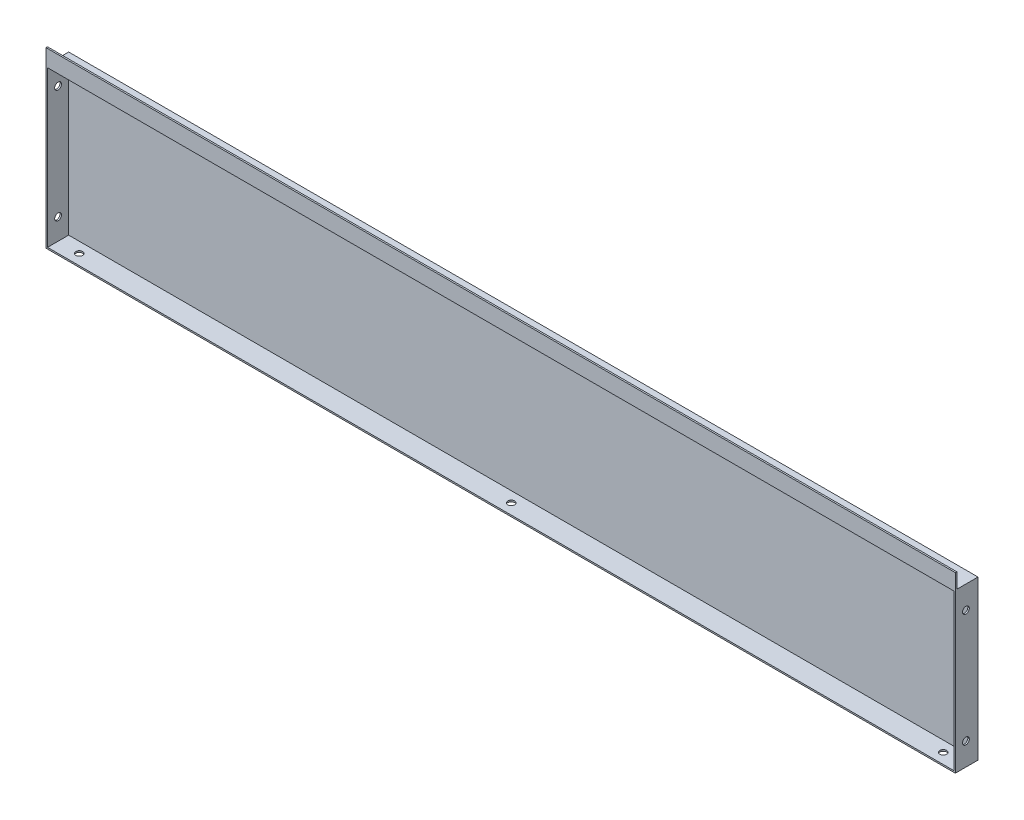
from build123d import *

# Parameters (mm, degrees)
SKETCH_1_W               = 1204
SKETCH_1_H               = 210
EXTRUDE_1_DEPTH          = 30
SHELL_1_T                = -2
SKETCH_2_W               = 1204
SKETCH_2_H               = 20
EXTRUDE_2_DEPTH          = 2
CUT_EXTRUDE_1_DEPTH      = 1477
CUT_EXTRUDE_1_DEPTH_BACK = 116
SKETCH_3_R               = 4.5
SKETCH_4_R               = 4.5
CUT_EXTRUDE_2_DEPTH      = 116


with BuildPart() as part:
    # 草图1 → 凸台-拉伸1 (new body)
    with BuildSketch(Plane.XY):
        with Locations((602, 105)):
            Rectangle(SKETCH_1_W, SKETCH_1_H)
    extrude(amount=EXTRUDE_1_DEPTH)

    # 抽壳1
    shell_1_openings = [part.faces().sort_by_distance(p)[0] for p in [
        (602, 105, 30),
    ]]
    offset(amount=SHELL_1_T, openings=shell_1_openings, kind=Kind.INTERSECTION)

    # 草图2 → 凸台-拉伸2 (add)
    with BuildSketch(Plane.XY.offset(30)):
        with Locations((602, 220)):
            Rectangle(SKETCH_2_W, SKETCH_2_H)
    extrude(amount=-EXTRUDE_2_DEPTH)

    # 草图3 → 切除-拉伸1 (cut, two sides: drawn at the far end of the back side and taken through both)
    with BuildSketch(Plane(origin=(2, 0, 0), x_dir=(0, 0, -1), z_dir=(1, 0, 0)).offset(-CUT_EXTRUDE_1_DEPTH_BACK)):
        with Locations(Location((-16, 180, 0), (0, 0, 180))):
            Circle(SKETCH_3_R)
        with Locations(Location((-16, 30, 0), (0, 0, 180))):
            Circle(SKETCH_3_R)
    extrude(amount=CUT_EXTRUDE_1_DEPTH + CUT_EXTRUDE_1_DEPTH_BACK, mode=Mode.SUBTRACT)

    # 草图4 → 切除-拉伸2 (cut)
    with BuildSketch(Plane(origin=(0, 2, 0), x_dir=(1, 0, 0), z_dir=(0, 1, 0))):
        with Locations(Location((30, -16, 0), (0, 0, 270))):
            Circle(SKETCH_4_R)
        with Locations(Location((1174, -16, 0), (0, 0, 270))):
            Circle(SKETCH_4_R)
        with Locations(Location((602, -16, 0), (0, 0, 270))):
            Circle(SKETCH_4_R)
    extrude(amount=-CUT_EXTRUDE_2_DEPTH, mode=Mode.SUBTRACT)


solid = part.part
